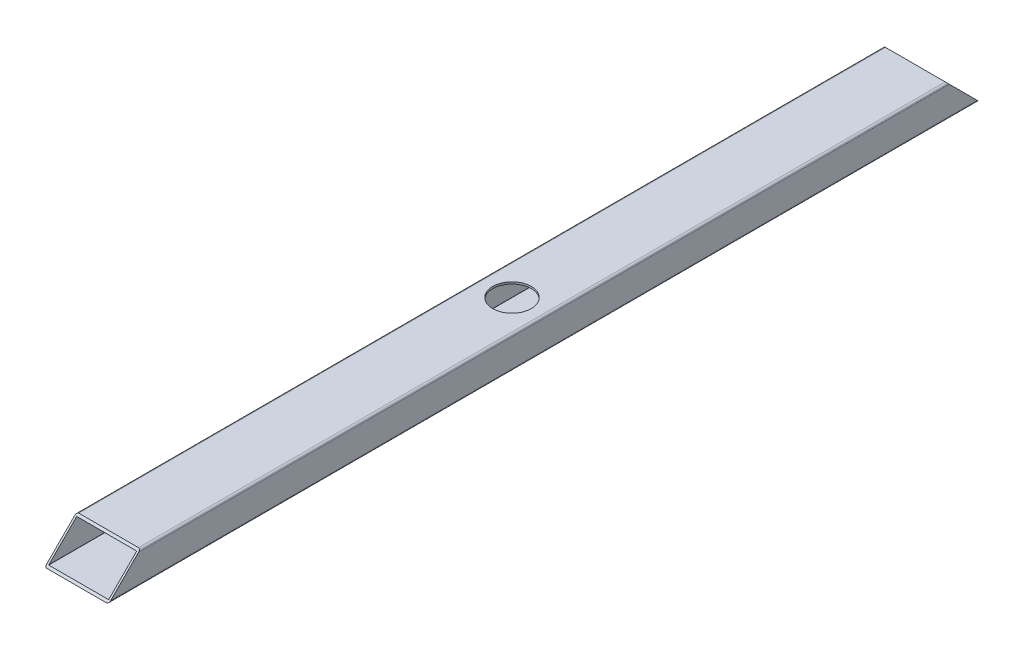
SolidWorks part; units mm, degrees
material "1023 碳钢板 (SS)"
ref_plane "前视基准面" through (0, 0, 0) normal (0, 0, 1) x (1, 0, 0)
ref_plane "上视基准面" through (0, 0, 0) normal (0, 1, 0) x (1, 0, 0)
ref_plane "右视基准面" through (0, 0, 0) normal (1, 0, 0) x (0, 0, -1)
sketch "草图1" plane through (0, 0, 0) normal (0, 0, 1) x (1, 0, 0)
  line L0 (-46.8, 22) -> (46.8, 22)
  line L1 (-46.8, 25) -> (46.8, 25)
  line L2 (-50, 21.8) -> (-50, -21.8)
  line L3 (-46.8, -25) -> (46.8, -25)
  line L4 (50, 21.8) -> (50, -21.8)
  line L5 (-50, 25) -> (50, -25) construction
  line L6 (-50, -25) -> (50, 25) construction
  line L7 (47, 21.8) -> (47, -21.8)
  line L8 (-46.8, -22) -> (46.8, -22)
  line L9 (-47, 21.8) -> (-47, -21.8)
  arc A0 (-50, -21.8) -> (-46.8, -25) centre (-46.8, -21.8) ccw
  arc A1 (46.8, -25) -> (50, -21.8) centre (46.8, -21.8) ccw
  arc A2 (46.8, 25) -> (50, 21.8) centre (46.8, 21.8) cw
  arc A3 (-46.8, 25) -> (-50, 21.8) centre (-46.8, 21.8) ccw
  arc A4 (46.8, 22) -> (47, 21.8) centre (46.8, 21.8) cw
  arc A5 (46.8, -22) -> (47, -21.8) centre (46.8, -21.8) ccw
  arc A6 (-47, -21.8) -> (-46.8, -22) centre (-46.8, -21.8) ccw
  arc A7 (-46.8, 22) -> (-47, 21.8) centre (-46.8, 21.8) ccw
  point P0 (0, 0)
  dimension "D3" = 3.2
  dimension "D1" = 100
  dimension "D2" = 50
  dimension "D4" = 3
extrude "凸台-拉伸1" add sketch "草图1" along normal blind 1400
sketch "草图2" plane through (50, 0, 0) normal (1, 0, 0) x (0, 0, -1)
  line L0 (-1318.4101, 25) -> (-1368.4101, -25)
  line L1 (-1400, 25) -> (0, 25) construction
  line L2 (-1400, -25) -> (0, -25) construction
  line L3 (-54.4101, 25) -> (-4.4101, -25)
  line L4 (-1318.4101, 25) -> (-1552.7564, 36.5074)
  line L5 (-1552.7564, 36.5074) -> (-1510.1517, -71.5631)
  line L6 (-1510.1517, -71.5631) -> (-1368.4101, -25)
  line L7 (-54.4101, 25) -> (0, 63.5251)
  line L8 (0, 63.5251) -> (119.219, 25)
  line L9 (119.219, 25) -> (74.0549, -20.1641)
  line L10 (74.0549, -20.1641) -> (36.9927, -46.406)
  line L11 (36.9927, -46.406) -> (-4.4101, -25)
  dimension "D1" = 45
  dimension "D2" = 45
  dimension "D3" = 1364
extrude "切除-拉伸1" cut sketch "草图2" against normal blind 1400
sketch "草图3" plane through (0, 25, 0) normal (0, 1, 0) x (1, 0, 0)
  circle A0 centre (0, -686.4101) radius 30.15
  dimension "D1" = 60.3
extrude "切除-拉伸2" cut sketch "草图3" against normal blind 218
